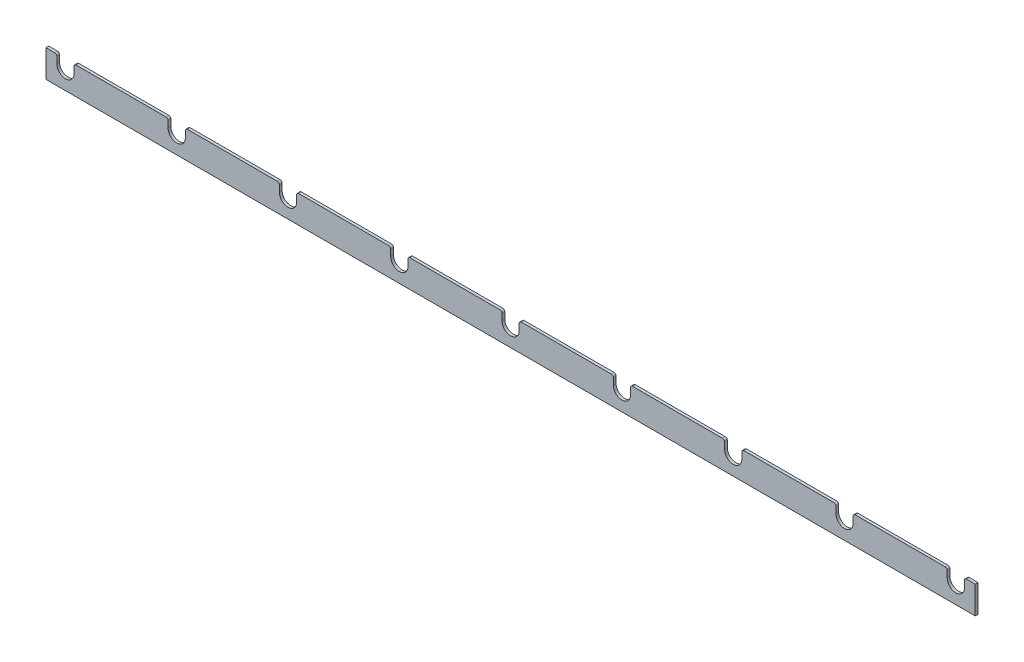
SolidWorks part; units mm, degrees
material "1023 Carbon Steel Plate (SS)"
ref_plane "Front Plane" through (0, 0, 0) normal (0, 0, 1) x (1, 0, 0)
ref_plane "Top Plane" through (0, 0, 0) normal (0, 1, 0) x (1, 0, 0)
ref_plane "Right Plane" through (0, 0, 0) normal (1, 0, 0) x (0, 0, -1)
sketch "Sketch1" plane through (0, 0, 0) normal (0, 0, 1) x (1, 0, 0)
  line L1 (675, 20) -> (-675, 20)
  line L2 (675, 20) -> (675, -20)
  line L3 (675, -20) -> (-675, -20)
  line L4 (-675, 20) -> (-675, -20)
  line L5 (675, 20) -> (-675, -20) construction
  line L6 (675, -20) -> (-675, 20) construction
  point P0 (0, 0)
  dimension "D1" = 1350
  dimension "D2" = 40
extrude "Boss-Extrude1" add sketch "Sketch1" along normal blind 4
sketch "Sketch2" plane through (0, 0, 4) normal (0, 0, 1) x (1, 0, 0)
  line L0 (675, 20) -> (-675, 20) construction
  line L1 (-675, 20) -> (-675, -20) construction
  line L2 (-659.3, 7.5) -> (-659.3, 20)
  line L3 (-659.3, 20) -> (-634.3, 20)
  line L4 (-634.3, 20) -> (-634.3, 7.5)
  line L5 (-497.6, 7.5) -> (-497.6, 20)
  line L6 (-497.6, 20) -> (-472.6, 20)
  line L7 (-472.6, 20) -> (-472.6, 7.5)
  line L8 (-335.9, 7.5) -> (-335.9, 20)
  line L9 (-335.9, 20) -> (-310.9, 20)
  line L10 (-310.9, 20) -> (-310.9, 7.5)
  line L11 (-174.2, 7.5) -> (-174.2, 20)
  line L12 (-174.2, 20) -> (-149.2, 20)
  line L13 (-149.2, 20) -> (-149.2, 7.5)
  line L14 (-12.5, 7.5) -> (-12.5, 20)
  line L15 (-12.5, 20) -> (12.5, 20)
  line L16 (12.5, 20) -> (12.5, 7.5)
  line L17 (149.2, 7.5) -> (149.2, 20)
  line L18 (149.2, 20) -> (174.2, 20)
  line L19 (174.2, 20) -> (174.2, 7.5)
  line L20 (310.9, 7.5) -> (310.9, 20)
  line L21 (310.9, 20) -> (335.9, 20)
  line L22 (335.9, 20) -> (335.9, 7.5)
  line L23 (472.6, 7.5) -> (472.6, 20)
  line L24 (472.6, 20) -> (497.6, 20)
  line L25 (497.6, 20) -> (497.6, 7.5)
  line L26 (634.3, 7.5) -> (634.3, 20)
  line L27 (634.3, 20) -> (659.3, 20)
  line L28 (659.3, 20) -> (659.3, 7.5)
  arc A0 (-659.3, 7.5) -> (-634.3, 7.5) centre (-646.8, 7.5) ccw
  arc A1 (-497.6, 7.5) -> (-472.6, 7.5) centre (-485.1, 7.5) ccw
  arc A2 (-335.9, 7.5) -> (-310.9, 7.5) centre (-323.4, 7.5) ccw
  arc A3 (-174.2, 7.5) -> (-149.2, 7.5) centre (-161.7, 7.5) ccw
  arc A4 (-12.5, 7.5) -> (12.5, 7.5) centre (0, 7.5) ccw
  arc A5 (149.2, 7.5) -> (174.2, 7.5) centre (161.7, 7.5) ccw
  arc A6 (310.9, 7.5) -> (335.9, 7.5) centre (323.4, 7.5) ccw
  arc A7 (472.6, 7.5) -> (497.6, 7.5) centre (485.1, 7.5) ccw
  arc A8 (634.3, 7.5) -> (659.3, 7.5) centre (646.8, 7.5) ccw
  dimension "D2" = 25
  dimension "D3" = 28.2
  dimension "D1" = 12.5
  dimension "D4" = 9
extrude "Cut-Extrude1" cut sketch "Sketch2" against normal blind 4
fillet "Fillet1" radius 3 18 edges at (-634.3, 20, 2) (-659.3, 20, 2) (659.3, 20, 2) (634.3, 20, 2) (497.6, 20, 2) (472.6, 20, 2) (335.9, 20, 2) (310.9, 20, 2) (174.2, 20, 2) (149.2, 20, 2) (12.5, 20, 2) (-12.5, 20, 2) (-149.2, 20, 2) (-174.2, 20, 2) (-310.9, 20, 2) (-335.9, 20, 2) (-472.6, 20, 2) (-497.6, 20, 2)
